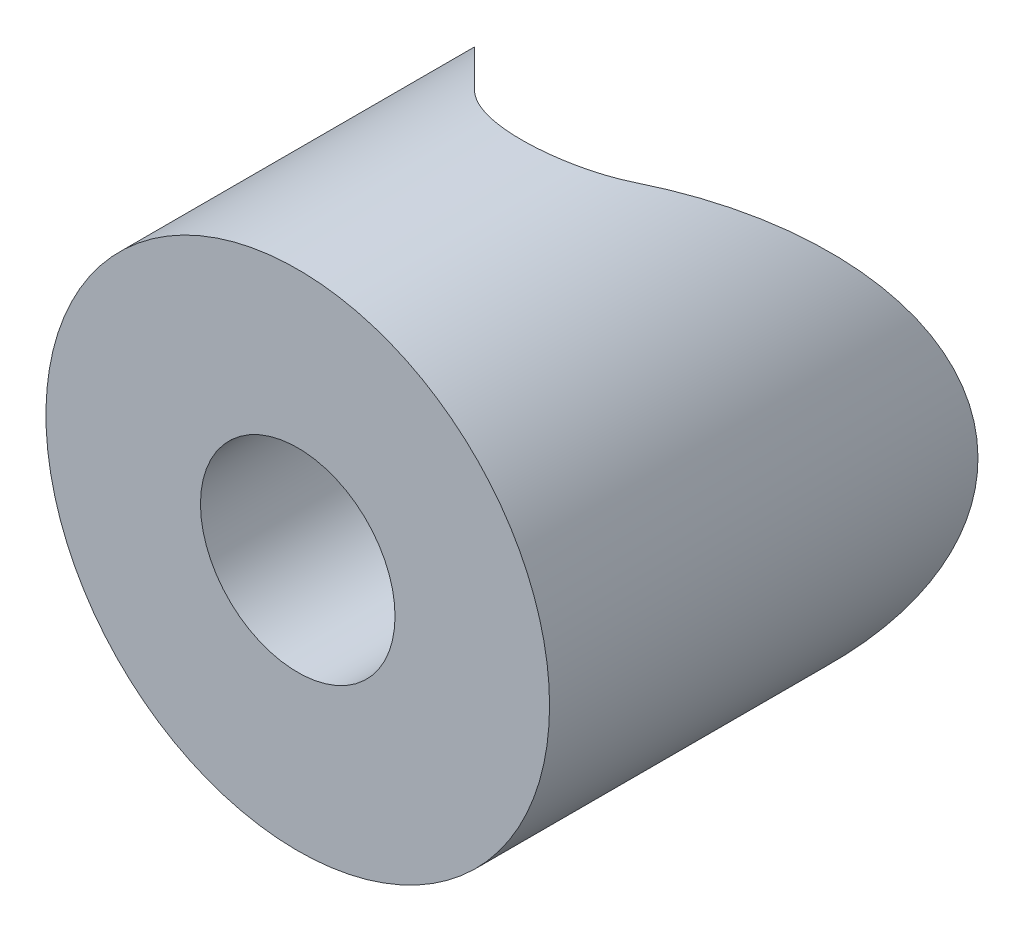
from build123d import *

# Parameters (mm, degrees)
SKETCH1_R              = 11
BOSS_EXTRUDE1_DEPTH    = 19
M10_TAPPED_HOLE1_D     = 8.5
M10_TAPPED_HOLE1_DEPTH = 24.5
M10_TAPPED_HOLE1_TIP   = 2.553657631
CUT_EXTRUDE1_DEPTH     = 12.5


with BuildPart() as part:
    # Sketch1 → Boss-Extrude1 (new body)
    with BuildSketch(Plane.XY):
        Circle(SKETCH1_R)
    extrude(amount=BOSS_EXTRUDE1_DEPTH)

    # M10 Tapped Hole1
    with Locations(Plane.XY.offset(19)):
        with Locations((0, 0)):
            Hole(M10_TAPPED_HOLE1_D / 2, depth=M10_TAPPED_HOLE1_DEPTH)
            with Locations((0, 0, -(M10_TAPPED_HOLE1_DEPTH + M10_TAPPED_HOLE1_TIP / 2))):  # 118° drill point
                Cone(0, M10_TAPPED_HOLE1_D / 2, M10_TAPPED_HOLE1_TIP, mode=Mode.SUBTRACT)

    # Sketch4 → Cut-Extrude1 (cut, symmetric)
    with BuildSketch(Plane(origin=(0, 0, 0), x_dir=(1, 0, 0), z_dir=(0, 1, 0))):
        with BuildLine():
            Line((3.535533906, -7.748737342), (28.284271247, 17))
            Line((28.284271247, 17), (0, 45.284271247))
            Line((0, 45.284271247), (-28.284271247, 17))
            Line((-28.284271247, 17), (-3.535533906, -7.748737342))
            ThreePointArc((-3.535533906, -7.748737342), (0, -9.213203436), (3.535533906, -7.748737342))
        make_face()
    extrude(amount=CUT_EXTRUDE1_DEPTH, both=True, mode=Mode.SUBTRACT)


solid = part.part
